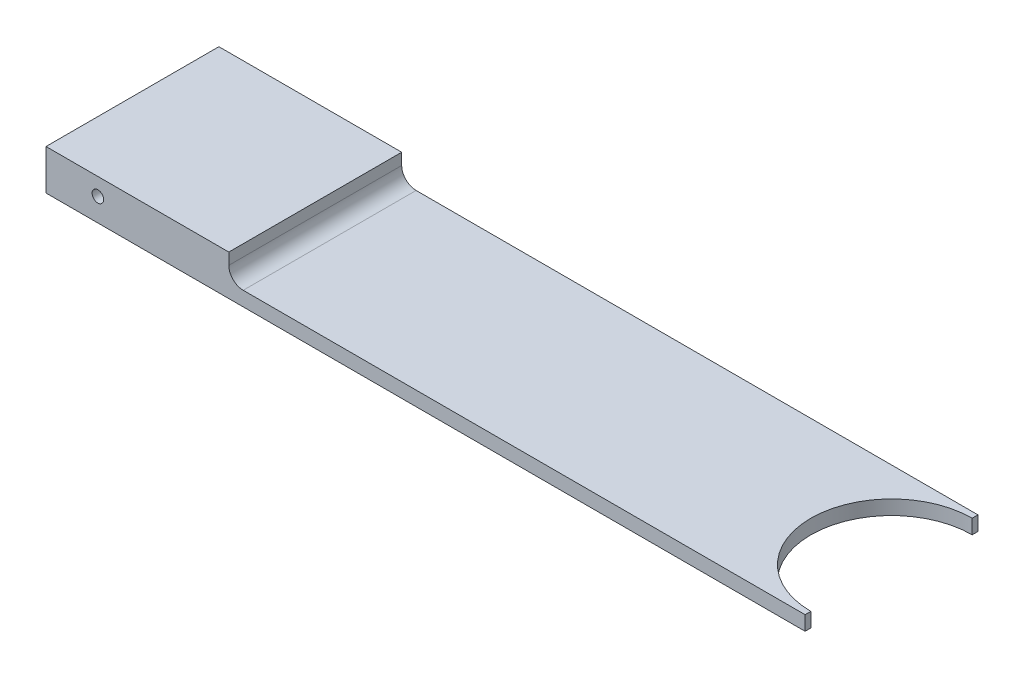
from build123d import *

# Parameters (mm, degrees)
BOSS_EXTRUDE2_DEPTH = 2.5
SKETCH5_W           = 63.43934648
SKETCH5_H           = 13.991199956
BOSS_EXTRUDE3_DEPTH = 30
FILLET1_R           = 5
SKETCH6_R           = 2
CUT_EXTRUDE1_DEPTH  = 162.963105911


with BuildPart() as part:
    # Sketch2 → Boss-Extrude2 (new, symmetric)
    with BuildSketch(Plane(origin=(0, 0, 0), x_dir=(1, 0, 0), z_dir=(0, 1, 0))):
        with BuildLine():
            Line((-50, 30), (50, 30))
            Line((50, 30), (150, 30))
            Line((150, 30), (150, 28))
            ThreePointArc((150, 28), (122, 0), (150, -28))
            Line((150, -28), (150, -30))
            Line((150, -30), (50, -30))
            Line((50, -30), (-50, -30))
            Line((-50, -30), (-50, 30))
        make_face()
    extrude(amount=BOSS_EXTRUDE2_DEPTH, both=True)

    # Sketch5 → Boss-Extrude3 (add, symmetric)
    with BuildSketch(Plane.XY):
        with Locations((-81.71967324, 4.495599978)):
            Rectangle(SKETCH5_W, SKETCH5_H)
    extrude(amount=BOSS_EXTRUDE3_DEPTH, both=True)

    # Fillet1
    fillet1_edges = [part.edges().sort_by_distance(p)[0] for p in [
        (-50, 2.5, 0),
    ]]
    fillet(fillet1_edges, radius=FILLET1_R)

    # Sketch6 → Cut-Extrude1 (cut, through all)
    with BuildSketch(Plane.XY.offset(30)):
        with Locations((-95.43934648, 5.491199956)):
            Circle(SKETCH6_R)
    extrude(amount=-CUT_EXTRUDE1_DEPTH, mode=Mode.SUBTRACT)


solid = part.part
